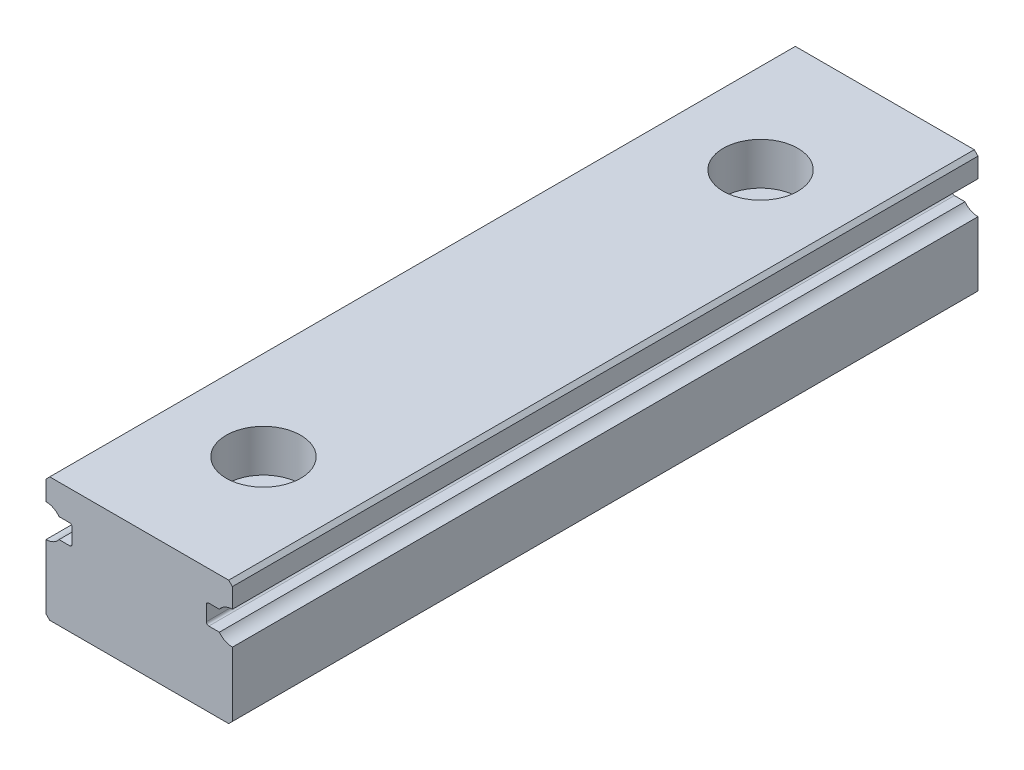
SolidWorks part; units mm, degrees
ref_plane "前视基准面" through (0, 0, 0) normal (0, 0, 1) x (1, 0, 0)
ref_plane "上视基准面" through (0, 0, 0) normal (0, 1, 0) x (1, 0, 0)
ref_plane "右视基准面" through (0, 0, 0) normal (1, 0, 0) x (0, 0, -1)
sketch "草图2" plane through (0, 0, 0) normal (0, 0, 1) x (1, 0, 0)
  line B0 (7.5, 9.7) -> (7.2, 10)
  line B1 (7.2, 10) -> (-7.2, 10)
  line B2 (-7.2, 10) -> (-7.5, 9.7)
  line B3 (-7.5, 9.7) -> (-7.5, 8.12)
  line B4 (-6.45, 7.6) -> (-5.6, 7.6)
  line B5 (-5.4, 7.4) -> (-5.4, 6.2)
  line B6 (-5.6, 6) -> (-6.45, 6)
  line B7 (-7.5, 5.48) -> (-7.5, 0.3)
  line B8 (-7.5, 0.3) -> (-7.2, 0)
  line B9 (-7.2, 0) -> (7.2, 0)
  line B10 (7.2, 0) -> (7.5, 0.3)
  line B11 (7.5, 0.3) -> (7.5, 5.48)
  line B12 (6.45, 6) -> (5.6, 6)
  line B13 (5.4, 6.2) -> (5.4, 7.4)
  line B14 (5.6, 7.6) -> (6.45, 7.6)
  line B15 (7.5, 8.12) -> (7.5, 9.7)
  arc B16 (-6.45, 7.6) -> (-7.5, 8.12) centre (-7.5, 6.8) ccw
  arc B17 (-5.4, 7.4) -> (-5.6, 7.6) centre (-5.6, 7.4) ccw
  arc B18 (-5.6, 6) -> (-5.4, 6.2) centre (-5.6, 6.2) ccw
  arc B19 (-7.5, 5.48) -> (-6.45, 6) centre (-7.5, 6.8) ccw
  arc B20 (6.45, 6) -> (7.5, 5.48) centre (7.5, 6.8) ccw
  arc B21 (5.4, 6.2) -> (5.6, 6) centre (5.6, 6.2) ccw
  arc B22 (5.6, 7.6) -> (5.4, 7.4) centre (5.6, 7.4) ccw
  arc B23 (7.5, 8.12) -> (6.45, 7.6) centre (7.5, 6.8) ccw
sketch_block_instance "块1-1"
sketch_block "块1"
extrude "凸台-拉伸1" add sketch "草图2" along normal mid plane 60
sketch "草图3" plane through (0, 10, 0) normal (0, 1, 0) x (1, 0, 0)
  line L0 (0, -30) -> (0, 30) construction
  line L1 (7.2, -30) -> (-7.2, -30) construction
  line L2 (7.2, 30) -> (-7.2, 30) construction
hole_wizard "打孔尺寸(%根据)内六角圆柱头螺钉的类型1" positions "3D草图1" profile "草图4" counterbore size "M3" standard "GB" end condition up to next
sketch3d "3D草图1"
  line L0 (0, 10, 30) -> (0, 10, -30) construction
  line L1 (7.2, 10, 30) -> (-7.2, 10, 30) construction
  point P0 (0, 10, 20)
  dimension "D1" = 10
sketch "草图4" plane through (0, 10, 20) normal (1, 0, 0) x (0, 0, 1)
  line L0 (0, 0) -> (0, 10.001)
  line L1 (0, 10.001) -> (1.7, 10.001)
  line L3 (1.7, 10.001) -> (1.7, 3.4)
  line L4 (1.7, 3.4) -> (3, 3.4)
  line L5 (3, 3.4) -> (3, 0)
  line L7 (3, 0) -> (0, 0)
  line L11 (0, -6.35) -> (0, 107.95) construction
  dimension "通孔孔直径" = 3.4
  dimension "通孔孔深度" = 10.001
  dimension "柱形沉头孔直径" = 6
  dimension "柱形沉头孔深度" = 3.4
pattern_linear "阵列(线性)1" count 2 spacing 40 along (0, 0, -1) of "打孔尺寸(%根据)内六角圆柱头螺钉的类型1"
